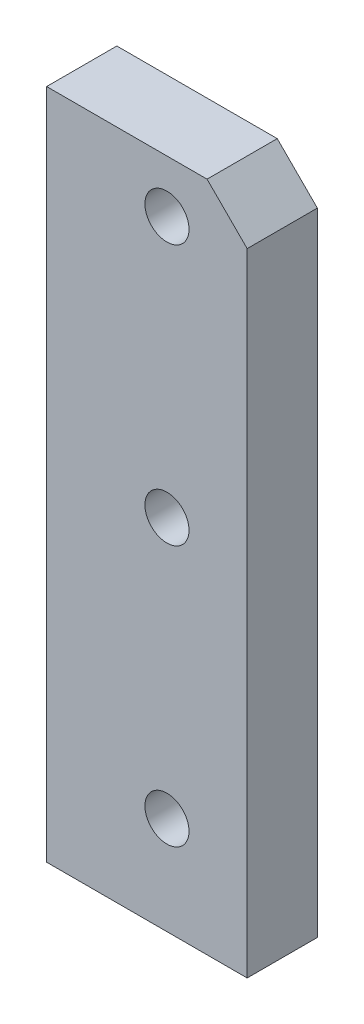
from build123d import *

# Parameters (mm, degrees)
SKETCH_1_W               = 100
SKETCH_1_H               = 335
EXTRUDE_1_DEPTH          = 35
CHAMFER_1_SIZE           = 20
CUT_EXTRUDE_1_DEPTH      = 179.27296486
CUT_EXTRUDE_1_DEPTH_BACK = 179.27296486
SKETCH_2_R               = 11


with BuildPart() as part:
    # 草图1 → 凸台-拉伸1 (new body)
    with BuildSketch(Plane.XY):
        Rectangle(SKETCH_1_W, SKETCH_1_H)
    extrude(amount=EXTRUDE_1_DEPTH)

    # 倒角1
    chamfer_1_edges = [part.edges().sort_by_distance(p)[0] for p in [
        (50, 167.5, 17.5),
    ]]
    chamfer(chamfer_1_edges, length=CHAMFER_1_SIZE)

    # 草图2 → 切除-拉伸1 (cut, two sides: drawn at the far end of the back side and taken through both)
    with BuildSketch(Plane.XY.offset(35).offset(-CUT_EXTRUDE_1_DEPTH_BACK)):
        with Locations((10, 141.327613457)):
            Circle(SKETCH_2_R)
        with Locations((10, -118.672386543)):
            Circle(SKETCH_2_R)
        with Locations((10, 11.327613457)):
            Circle(SKETCH_2_R)
    extrude(amount=CUT_EXTRUDE_1_DEPTH + CUT_EXTRUDE_1_DEPTH_BACK, mode=Mode.SUBTRACT)


solid = part.part
